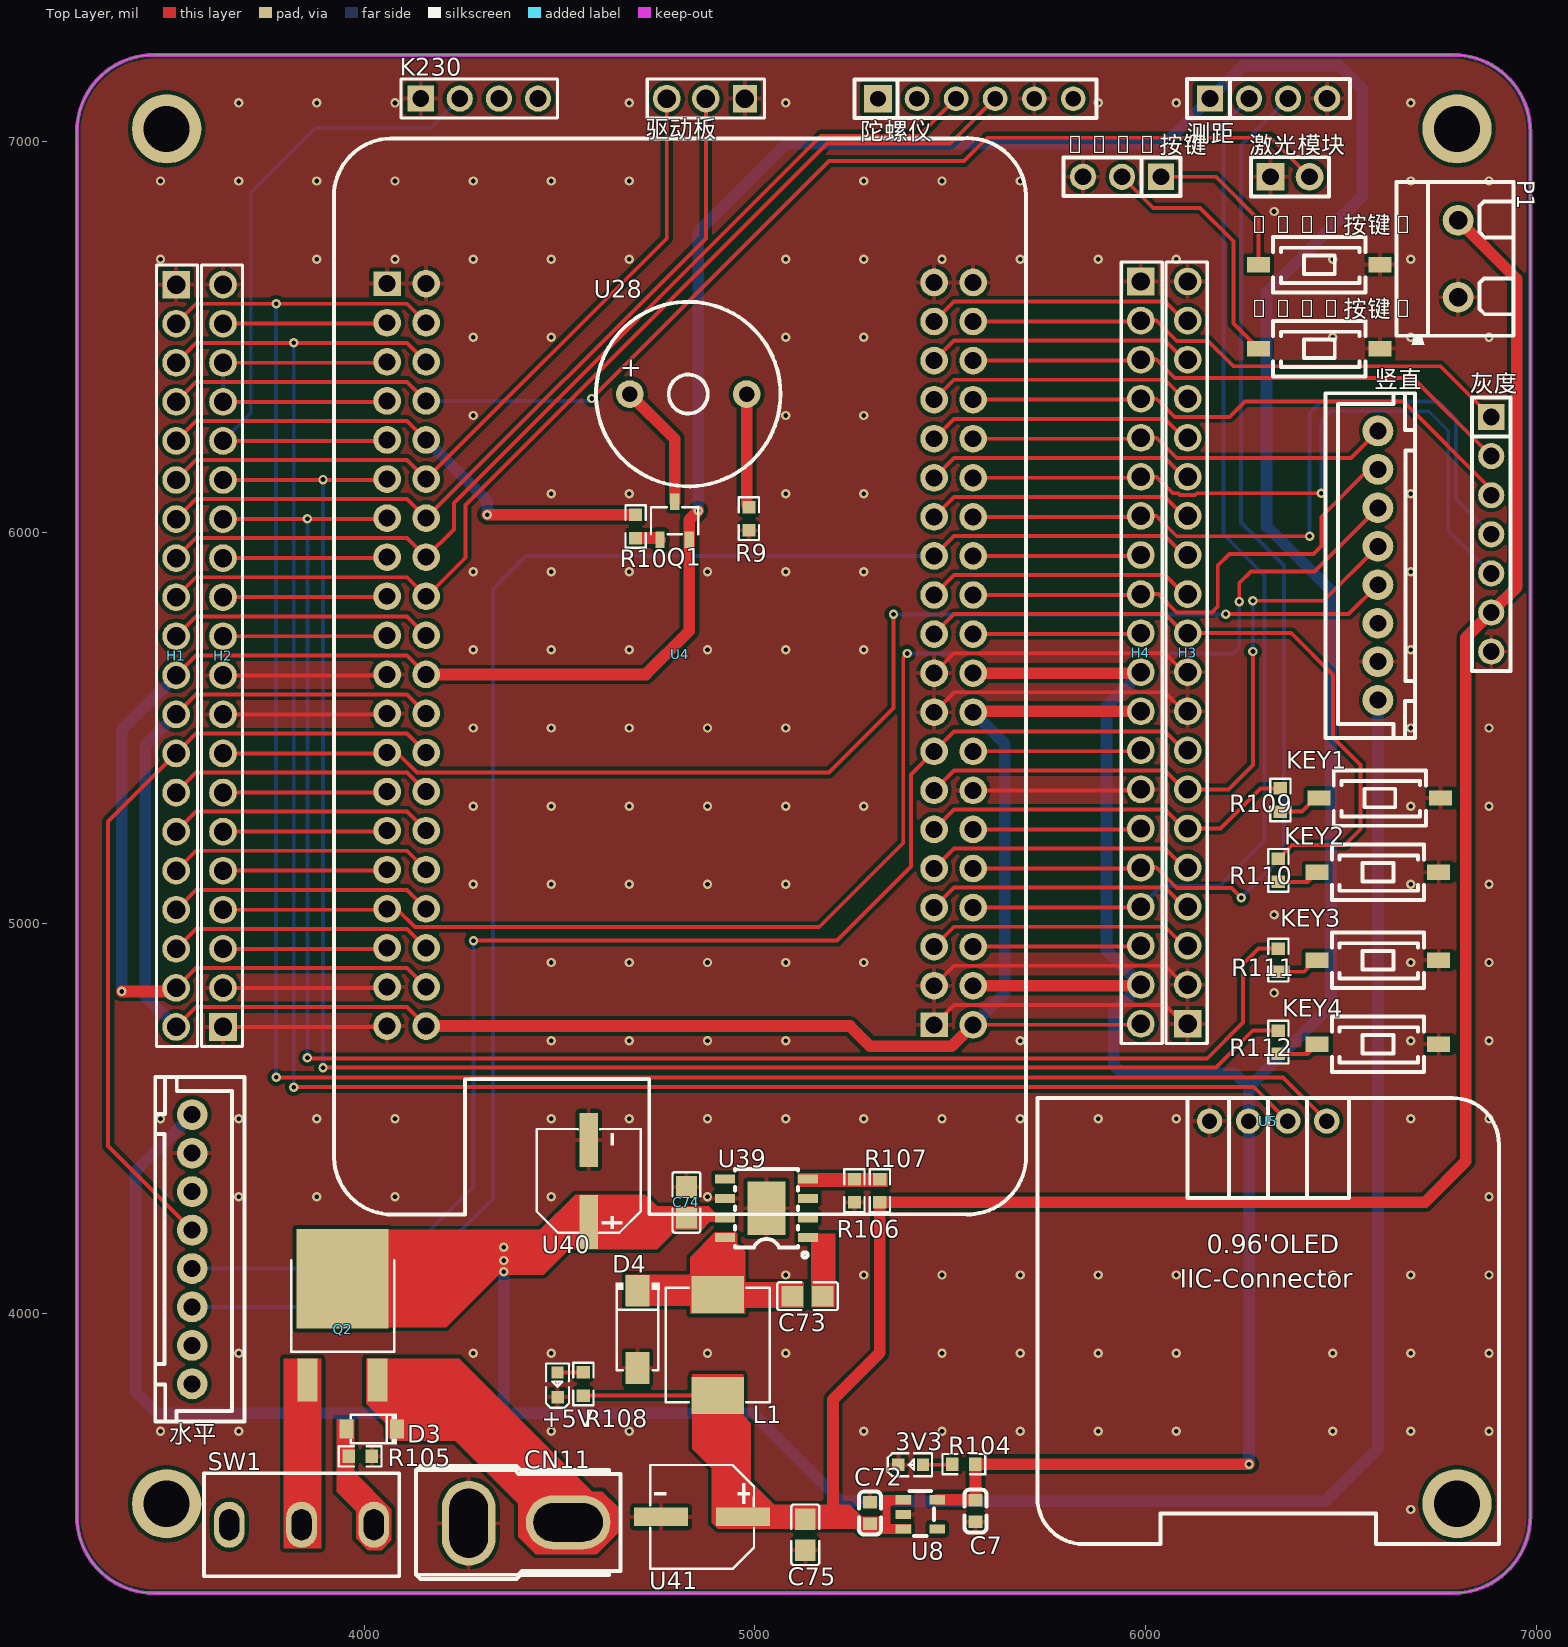
[diagram p0: Top Layer view]
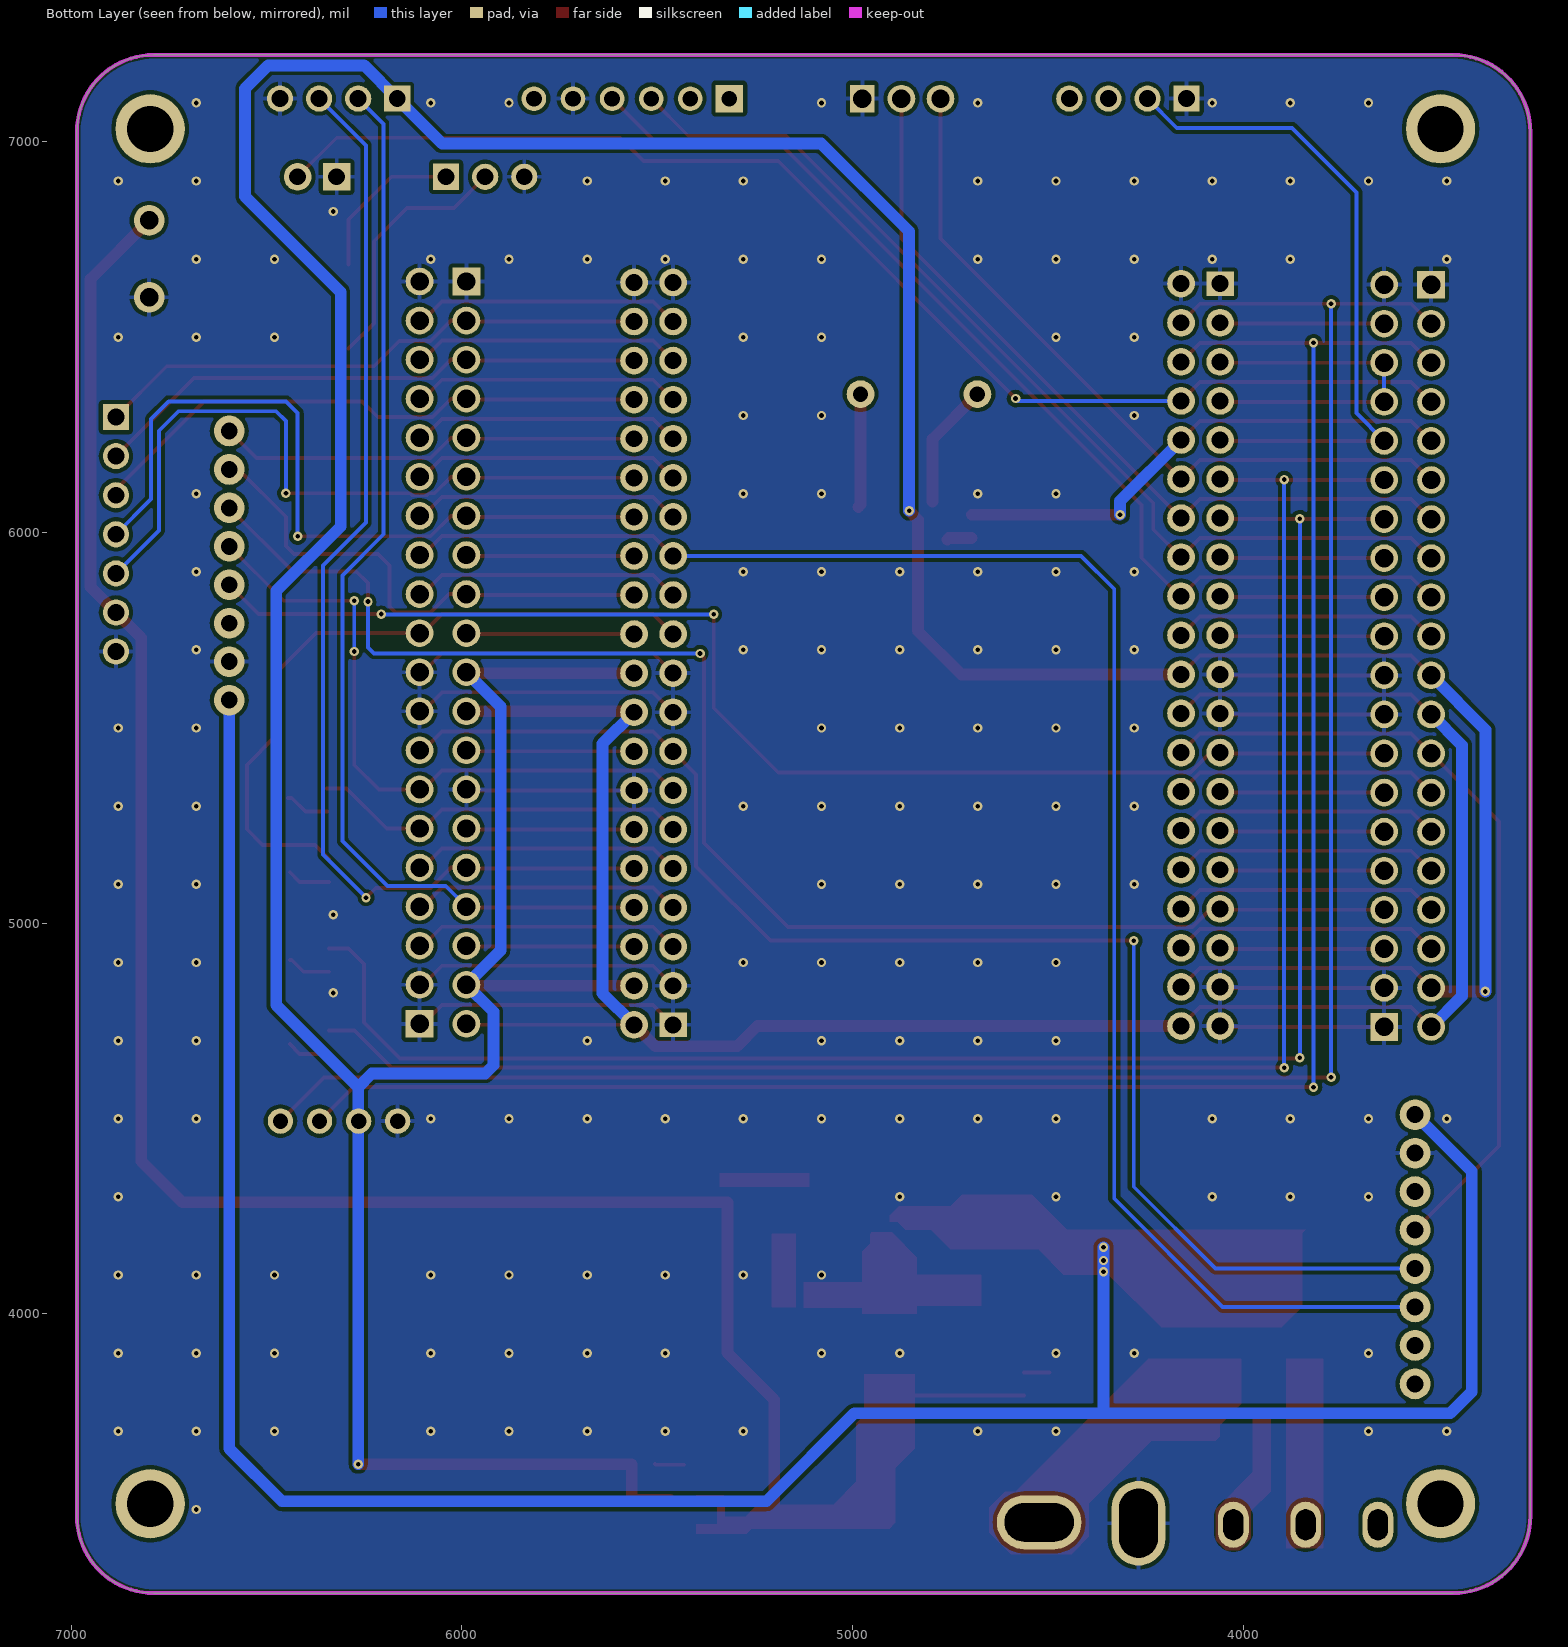
[diagram p1: Bottom Layer view, seen from below]
# Altium PCB MISC49883.pcbdoc
Units mil, origin at the board's own origin, x right, y up, seen from the top; angles counter-clockwise.
Board outline 3720 x 3937 mil, 2 copper layers (Top Layer, Bottom Layer), stack 62.206 mil thick; 52 components, 82 nets, 300 pads, 183 vias.

## Layer stack, top to bottom
Top Solder Mask Layer: solder mask 0.394, Dk 3.3
Top Layer: signal copper 1.379
Dielectric1: surface 59.449, FR4, Dk 4.5
Bottom Layer: signal copper 1.378
Bottom Solder Mask Layer: solder mask 0.394, Dk 3.3

## Board outline
3461.9,7222 ccw(c3461.9,7025.1) 3265,7025.1 3265,3481.9 ccw(c3461.9,3481.9) 3461.9,3285 6788.1,3285 ccw(c6788.1,3481.9) 6985,3481.9 6985,7025.1 ccw(c6788.1,7025.1) 6788.1,7222 3461.9,7222

## Design rules (kind name [scope] priority, off if disabled: settings)
BoardOutlineClearance copperThickness2oz_1 [All] p2 off: genericclearance=7.99 ignorepadtopadclearanceinfootprint=FALSE except(0: Arc-SplitContinuation Track-SplitContinuation SMDPad-SplitContinuation THPad-SplitContinuation Via-SplitContinuation Fill-SplitContinuation Region-SplitContinuation Poly-SplitContinuation Text-SplitContinuation Hole-SplitContinuation; 5.98: Arc-CutoutEdge Track-CutoutEdge SMDPad-CutoutEdge THPad-CutoutEdge Via-CutoutEdge Text-CutoutEdge; 6.9: Hole-OutlineEdge Hole-CutoutEdge; 10: Poly-OutlineEdge Poly-CutoutEdge; 11.81: Arc-OutlineEdge Track-OutlineEdge SMDPad-OutlineEdge THPad-OutlineEdge Via-OutlineEdge Fill-OutlineEdge Region-OutlineEdge Text-OutlineEdge Fill-CutoutEdge Region-CutoutEdge)
BoardOutlineClearance Plane_innerPlane_1 [All] p4 off: genericclearance=4.02 ignorepadtopadclearanceinfootprint=FALSE except(0: Arc-SplitContinuation Track-SplitContinuation SMDPad-SplitContinuation THPad-SplitContinuation Via-SplitContinuation Fill-SplitContinuation Region-SplitContinuation Poly-SplitContinuation Text-SplitContinuation Hole-SplitContinuation; 5.98: Arc-CutoutEdge Track-CutoutEdge SMDPad-CutoutEdge THPad-CutoutEdge Via-CutoutEdge Text-CutoutEdge; 6.9: Hole-OutlineEdge Hole-CutoutEdge; 10: Poly-OutlineEdge Poly-CutoutEdge; 11.81: Arc-OutlineEdge Track-OutlineEdge SMDPad-OutlineEdge THPad-OutlineEdge Via-OutlineEdge Fill-OutlineEdge Region-OutlineEdge Text-OutlineEdge Fill-CutoutEdge Region-CutoutEdge)
BoardOutlineClearance Copper_copperRegion_1 [All] p6 off: genericclearance=4.02 ignorepadtopadclearanceinfootprint=FALSE except(0: Arc-SplitContinuation Track-SplitContinuation SMDPad-SplitContinuation THPad-SplitContinuation Via-SplitContinuation Fill-SplitContinuation Region-SplitContinuation Poly-SplitContinuation Text-SplitContinuation Hole-SplitContinuation; 5.98: Arc-CutoutEdge Track-CutoutEdge SMDPad-CutoutEdge THPad-CutoutEdge Via-CutoutEdge Text-CutoutEdge; 6.9: Hole-OutlineEdge Hole-CutoutEdge; 10: Poly-OutlineEdge Poly-CutoutEdge; 11.81: Arc-OutlineEdge Track-OutlineEdge SMDPad-OutlineEdge THPad-OutlineEdge Via-OutlineEdge Fill-OutlineEdge Region-OutlineEdge Text-OutlineEdge Fill-CutoutEdge Region-CutoutEdge)
BoardOutlineClearance Copper_copperRegion_copperThickness1oz_1 [All] p8 off: genericclearance=4.02 ignorepadtopadclearanceinfootprint=FALSE except(0: Arc-SplitContinuation Track-SplitContinuation SMDPad-SplitContinuation THPad-SplitContinuation Via-SplitContinuation Fill-SplitContinuation Region-SplitContinuation Poly-SplitContinuation Text-SplitContinuation Hole-SplitContinuation; 5.98: Arc-CutoutEdge Track-CutoutEdge SMDPad-CutoutEdge THPad-CutoutEdge Via-CutoutEdge Text-CutoutEdge; 6.9: Hole-OutlineEdge Hole-CutoutEdge; 10: Poly-OutlineEdge Poly-CutoutEdge; 11.81: Arc-OutlineEdge Track-OutlineEdge SMDPad-OutlineEdge THPad-OutlineEdge Via-OutlineEdge Fill-OutlineEdge Region-OutlineEdge Text-OutlineEdge Fill-CutoutEdge Region-CutoutEdge)
BoardOutlineClearance Copper_copperRegion_Copper_copperRegion_1 [All] p10 off: genericclearance=4.02 ignorepadtopadclearanceinfootprint=FALSE except(0: Arc-SplitContinuation Track-SplitContinuation SMDPad-SplitContinuation THPad-SplitContinuation Via-SplitContinuation Fill-SplitContinuation Region-SplitContinuation Poly-SplitContinuation Text-SplitContinuation Hole-SplitContinuation; 5.98: Arc-CutoutEdge Track-CutoutEdge SMDPad-CutoutEdge THPad-CutoutEdge Via-CutoutEdge Text-CutoutEdge; 6.9: Hole-OutlineEdge Hole-CutoutEdge; 10: Poly-OutlineEdge Poly-CutoutEdge; 11.81: Arc-OutlineEdge Track-OutlineEdge SMDPad-OutlineEdge THPad-OutlineEdge Via-OutlineEdge Fill-OutlineEdge Region-OutlineEdge Text-OutlineEdge Fill-CutoutEdge Region-CutoutEdge)
BoardOutlineClearance copperThickness1oz_1 [All] p12: genericclearance=4.02 ignorepadtopadclearanceinfootprint=FALSE except(0: Arc-SplitContinuation Track-SplitContinuation SMDPad-SplitContinuation THPad-SplitContinuation Via-SplitContinuation Fill-SplitContinuation Region-SplitContinuation Poly-SplitContinuation Text-SplitContinuation Hole-SplitContinuation; 5.98: Arc-CutoutEdge Track-CutoutEdge SMDPad-CutoutEdge THPad-CutoutEdge Via-CutoutEdge Text-CutoutEdge; 6.9: Hole-OutlineEdge Hole-CutoutEdge; 10: Poly-OutlineEdge Poly-CutoutEdge; 11.81: Arc-OutlineEdge Track-OutlineEdge SMDPad-OutlineEdge THPad-OutlineEdge Via-OutlineEdge Fill-OutlineEdge Region-OutlineEdge Text-OutlineEdge Fill-CutoutEdge Region-CutoutEdge)
Clearance copperThickness2oz [All] p1 off: gap=7.99 ignorepadtopadclearanceinfootprint=FALSE except(5.98: SMDPad-Track SMDPad-SMDPad THPad-Track SMDPad-THPad THPad-THPad Track-Via SMDPad-Via THPad-Via Via-Via Fill-SMDPad Region-SMDPad Fill-THPad Region-THPad Fill-Via Region-Via Fill-Fill Fill-Region Region-Region Arc-Track Arc-SMDPad Arc-THPad Arc-Via Fill-Arc Region-Arc Arc-Arc Text-Track SMDPad-Text Text-THPad Text-Via Fill-Text Region-Text Arc-Text Text-Text; 6.9: Hole-Track Hole-SMDPad Hole-THPad Hole-Via Fill-Hole Region-Hole Hole-Arc Hole-Text; 10: Poly-Track Poly-SMDPad Poly-THPad Poly-Via Poly-Fill Poly-Region Poly-Poly Poly-Arc Poly-Text Poly-Hole; 11.81: Fill-Track Region-Track)
Clearance Plane_innerPlane [All] p3 off: gap=4.02 ignorepadtopadclearanceinfootprint=FALSE except(5.98: SMDPad-Track SMDPad-SMDPad THPad-Track SMDPad-THPad THPad-THPad Track-Via SMDPad-Via THPad-Via Via-Via Fill-SMDPad Region-SMDPad Fill-THPad Region-THPad Fill-Via Region-Via Fill-Fill Fill-Region Region-Region Arc-Track Arc-SMDPad Arc-THPad Arc-Via Fill-Arc Region-Arc Arc-Arc Text-Track SMDPad-Text Text-THPad Text-Via Fill-Text Region-Text Arc-Text Text-Text; 6.9: Hole-Track Hole-SMDPad Hole-THPad Hole-Via Fill-Hole Region-Hole Hole-Arc Hole-Text; 10: Poly-Track Poly-SMDPad Poly-THPad Poly-Via Poly-Fill Poly-Region Poly-Poly Poly-Arc Poly-Text Poly-Hole; 11.81: Fill-Track Region-Track)
Clearance Copper_copperRegion [All] p5 off: gap=4.02 ignorepadtopadclearanceinfootprint=FALSE except(5.98: SMDPad-Track SMDPad-SMDPad THPad-Track SMDPad-THPad THPad-THPad Track-Via SMDPad-Via THPad-Via Via-Via Fill-SMDPad Region-SMDPad Fill-THPad Region-THPad Fill-Via Region-Via Fill-Fill Fill-Region Region-Region Arc-Track Arc-SMDPad Arc-THPad Arc-Via Fill-Arc Region-Arc Arc-Arc Text-Track SMDPad-Text Text-THPad Text-Via Fill-Text Region-Text Arc-Text Text-Text; 6.9: Hole-Track Hole-SMDPad Hole-THPad Hole-Via Fill-Hole Region-Hole Hole-Arc Hole-Text; 10: Poly-Track Poly-SMDPad Poly-THPad Poly-Via Poly-Fill Poly-Region Poly-Poly Poly-Arc Poly-Text Poly-Hole; 11.81: Fill-Track Region-Track)
Clearance Copper_copperRegion_copperThickness1oz [All] p7 off: gap=4.02 ignorepadtopadclearanceinfootprint=FALSE except(5.98: SMDPad-Track SMDPad-SMDPad THPad-Track SMDPad-THPad THPad-THPad Track-Via SMDPad-Via THPad-Via Via-Via Fill-SMDPad Region-SMDPad Fill-THPad Region-THPad Fill-Via Region-Via Fill-Fill Fill-Region Region-Region Arc-Track Arc-SMDPad Arc-THPad Arc-Via Fill-Arc Region-Arc Arc-Arc Text-Track SMDPad-Text Text-THPad Text-Via Fill-Text Region-Text Arc-Text Text-Text; 6.9: Hole-Track Hole-SMDPad Hole-THPad Hole-Via Fill-Hole Region-Hole Hole-Arc Hole-Text; 10: Poly-Track Poly-SMDPad Poly-THPad Poly-Via Poly-Fill Poly-Region Poly-Poly Poly-Arc Poly-Text Poly-Hole; 11.81: Fill-Track Region-Track)
Clearance Copper_copperRegion_Copper_copperRegion [All] p9 off: gap=4.02 ignorepadtopadclearanceinfootprint=FALSE except(5.98: SMDPad-Track SMDPad-SMDPad THPad-Track SMDPad-THPad THPad-THPad Track-Via SMDPad-Via THPad-Via Via-Via Fill-SMDPad Region-SMDPad Fill-THPad Region-THPad Fill-Via Region-Via Fill-Fill Fill-Region Region-Region Arc-Track Arc-SMDPad Arc-THPad Arc-Via Fill-Arc Region-Arc Arc-Arc Text-Track SMDPad-Text Text-THPad Text-Via Fill-Text Region-Text Arc-Text Text-Text; 6.9: Hole-Track Hole-SMDPad Hole-THPad Hole-Via Fill-Hole Region-Hole Hole-Arc Hole-Text; 10: Poly-Track Poly-SMDPad Poly-THPad Poly-Via Poly-Fill Poly-Region Poly-Poly Poly-Arc Poly-Text Poly-Hole; 11.81: Fill-Track Region-Track)
Clearance copperThickness1oz [All] p11: gap=4.02 ignorepadtopadclearanceinfootprint=FALSE except(5.98: SMDPad-Track SMDPad-SMDPad THPad-Track SMDPad-THPad THPad-THPad Track-Via SMDPad-Via THPad-Via Via-Via Fill-SMDPad Region-SMDPad Fill-THPad Region-THPad Fill-Via Region-Via Fill-Fill Fill-Region Region-Region Arc-Track Arc-SMDPad Arc-THPad Arc-Via Fill-Arc Region-Arc Arc-Arc Text-Track SMDPad-Text Text-THPad Text-Via Fill-Text Region-Text Arc-Text Text-Text; 6.9: Hole-Track Hole-SMDPad Hole-THPad Hole-Via Fill-Hole Region-Hole Hole-Arc Hole-Text; 10: Poly-Track Poly-SMDPad Poly-THPad Poly-Via Poly-Fill Poly-Region Poly-Poly Poly-Arc Poly-Text Poly-Hole; 11.81: Fill-Track Region-Track)
DiffPairsRouting differentialPair [All] p1: maxlimit=6 minlimit=6 mostfreqgap=6 toplayer_minwidth=5 toplayer_prefwidth=10 toplayer_maxwidth=100 toplayer_mingap=6 toplayer_prefgap=6 toplayer_maxgap=6 bottomlayer_minwidth=5 bottomlayer_prefwidth=10 bottomlayer_maxwidth=100 bottomlayer_mingap=6 bottomlayer_prefgap=6 bottomlayer_maxgap=6 maxuncoupledlength=10
HoleToHoleClearance otherClearance [All] p1: gap=11.81 allowstackedmicrovias=TRUE
Length netLength [All] p1: minlimit=0 maxlimit=0
PasteMaskExpansion pasteMaskExpansion [All] p1: expansion=0
PlaneConnect innerPlane [All] p1: planeconnectstyle=Relief reliefexpansion=20 reliefentries=4 reliefconductorwidth=10 reliefairgap=10
PolygonConnect copperRegion_copperThickness1oz [All] p1 off: connectstyle=Relief reliefconductorwidth=10 reliefentries=4 polygonreliefangle="90 Angle" airgapwidth=10 via.connectstyle=Relief via.reliefconductorwidth=10 via.reliefentries=4 via.polygonreliefangle="90 Angle" via.airgapwidth=10
PolygonConnect copperRegion_Copper_copperRegion [All] p2 off: connectstyle=Relief reliefconductorwidth=10 reliefentries=4 polygonreliefangle="90 Angle" airgapwidth=10 via.connectstyle=Relief via.reliefconductorwidth=10 via.reliefentries=4 via.polygonreliefangle="90 Angle" via.airgapwidth=10
PolygonConnect copperRegion [All] p3: connectstyle=Relief reliefconductorwidth=10 reliefentries=4 polygonreliefangle="90 Angle" airgapwidth=10 via.connectstyle=Relief via.reliefconductorwidth=10 via.reliefentries=4 via.polygonreliefangle="90 Angle" via.airgapwidth=10
RoutingVias viaSize [All] p1: holewidth=12.01 width=24.02 viastyle="Through Hole" minholewidth=11.81 minwidth=19.68 maxholewidth=248.03 maxwidth=393.7
SolderMaskExpansion solderMaskExpansion [IsVia] p1: expansion=-1000 istentingtop=TRUE
SolderMaskExpansion solderMaskExpansion [All] p2: expansion=2 istentingtop=FALSE
Width copperThickness2oz_2 [All] p1 off: maxlimit=100 minlimit=8 preferedwidth=10
Width copperThickness1oz_2 [All] p2: maxlimit=100 minlimit=5 preferedwidth=10

## Components (designator, comment, footprint, x,y, rotation, side; value= is the part's Value field where it differs from the comment)
3V3 "" LED_0603 5401.02,3613.64 r0 top
+5V "" LED_0603 4495,3820 r90 top
C7 "1uF" C0603 5565,3495 r90 top
C72 "1uF" C0603 5295,3490 r270 top
C73 "100nF" C0805 5135,4045 r180 top
C74 "100nF" C0805 4825,4285 r270 top
C75 "100nF" C0805 5129.37,3434.37 r90 top
CN11 "AM-1015B-M" CONN-TH_AM-1015B-M 4395,3465 r0 top
D3 "BZT52C16" SOD-123_L2.7-W1.6-LS3.7-RD 4020,3705 r180 top
D4 "SS54" SMA_L4.4-W2.8-LS5.4-R-RD 4700,3960 r270 top
H1 "" HDR-TH_20P-P2.54-V-M-1 3519,5684 r270 top
H2 "" HDR-TH_20P-P2.54-V-M-1 3639,5684 r90 top
H3 "" HDR-TH_20P-P2.54-V-M-1 6108,5692 r90 top
H4 "" HDR-TH_20P-P2.54-V-M-1 5988,5692 r270 top
K230 "2.54*4 single row" HDR-TH_4P-P2.54-V-M-1 4295,7110 r0 top
K230按键 "K230 button" HDR-TH_3P-P2.54-V-M 5940,6910 r180 top
K230按键1 "Tact switch 3*6*2.5" SW-SMD_L6.0-W3.6-LS8.0 6445,6685 r0 top
K230按键2 "Tact switch 3*6*2.5" SW-SMD_L6.0-W3.6-LS8.0 6445,6470 r0 top
KEY1 "Tact switch 3*6*2.5" SW-SMD_L6.0-W3.6-LS8.0 6600,5320 r0 top
KEY2 "Tact switch 3*6*2.5" SW-SMD_L6.0-W3.6-LS8.0 6595,5130 r0 top
KEY3 "Tact switch 3*6*2.5" SW-SMD_L6.0-W3.6-LS8.0 6595,4905 r0 top
KEY4 "Tact switch 3*6*2.5" SW-SMD_L6.0-W3.6-LS8.0 6595,4690 r0 top
L1 "4.7uH" IND-SMD_L7.3-W6.6 4905,3920 r90 top
P1 "KF301-2P terminal block" CONN-TH_XY301V-A-5.0-2P 6800,6700 r270 top
Q1 "S8550" SOT-23-3_L2.9-W1.6-P1.90-LS2.8-BR 4795,6030 r270 top
Q2 "HY19P03D" TO-252-2_L6.6-W6.1-P4.57-LS9.9-TL-CW 3945,3960 r90 top
R9 "100Ω" R0603 4985,6035 r90 top
R10 "100Ω" R0603 4695,6015 r90 top
R104 "10K" R0603 5535,3615 r180 top
R105 "10kΩ" R0603 3990,3635 r180 top
R106 "3.24K" R0603 5255,4315 r90 top
R107 "10K" R0603 5320,4315 r270 top
R108 "4.7K" R0603 4561.29,3820.26 r270 top
R109 "100Ω" R0603 6345,5315 r90 top
R110 "100Ω" R0603 6340,5135 r90 top
R111 "100Ω" R0603 6340,4905 r90 top
R112 "100Ω" R0603 6340,4695 r90 top
SW1 "SS-12D10L5" SW-TH_SS-12D10L5 3840,3460 r180 top
U4 "" COMM-TH_LCKFB-TMX-MSPM0G3507 4809,5688 r0 top
U5 "" 0.96OLED_4P 6314,4493 r0 top
U8 "TLV75733PDBVR" SOT-23-5_L2.9-W1.6-P0.95-LS2.8-BL 5423.52,3486.48 r270 top
U28 "2.6kHz" BUZ-TH_BD12.0-P7.60-D0.6-FD 4829.7,6353.8 r0 top
U39 "TPS5430DDAR" ESOP-8_L4.9-W3.9-P1.27-LS6.0-TL-EP 5030,4270 r180 top
U40 "220uF" CAP-SMD_BD6.3-L6.6-W6.6-LS7.2-FD 4575,4340 r90 top
U41 "220uF" CAP-SMD_BD6.3-L6.6-W6.6-LS7.2-FD 4865,3480 r180 top
水平 "Horizontal" CONN-TH_8P-P2.50-XH2.54-8P 3560,4165 r90 top (schematic designator ˮƽ)
测距 "PM2.54-1*4" HDR-TH_4P-P2.54-V-F 6315,7110 r0 top
激光模块 "" HDR-TH_2P-P2.54-V-M-1 6370,6910 r0 top
灰度 "PZ2.54-1*7" HDR-TH_7P-P2.54-V-M 6885,5995 r270 top
竖直 "Vertical" CONN-TH_8P-P2.50-XH2.54-8P 6595,5915 r270 top
陀螺仪 "2.54-1*6P female" HDR-TH_6P-P2.54-V-F 5565.21,7110 r0 top
驱动板 "2.54mm-1*3P straight pin" HDR-TH_3P-P2.54-V-M-1 4874.68,7110 r180 top

## Footprints (in the part's own frame and the unit in brackets; to place one, negate y for a bottom-side part, rotate by r counter-clockwise, add the part's x,y. Pads: shape width x height; smd on the part's side, far side on the other; paste and mask are expansions set on the pad)
0.96OLED_4P [mm]
  round 1.65 hole 1 copper offset 0,0: 1(-3.81,-0.001) 2(-1.27,0.002) 3(1.27,0.002) 4(3.81,0.002)
  silkscreen extent -15,-27.5 15,1.5
BUZ-TH_BD12.0-P7.60-D0.6-FD [mm]
  round 1.8 hole 1: 1(-3.8,0) 2(3.8,0)
  silkscreen extent -6,-6 6,6
C0603 [mm]
  rect 0.8x0.9 smd: 1(-0.7,0) 2(0.7,0)
  silkscreen extent -1.39,-0.71 1.39,0.71
C0805 [mm]
  rect 1.41x1.35 smd paste-100 mask+0.051: 1(-1,0) 2(1,0)
  silkscreen extent -1.96,-0.9 1.96,0.9
CAP-SMD_BD6.3-L6.6-W6.6-LS7.2-FD [mm]
  rect 3.5x1.2 smd: 1(-2.67,0) 2(2.67,0)
  silkscreen extent -3.38,-3.38 3.38,3.38
COMM-TH_LCKFB-TMX-MSPM0G3507 [mm]
  rect 1.8x1.575 hole 1.1: 1(-19.05,24.09) 41(16.51,-24.09)
  round 1.8 hole 1.1: 2(-16.51,24.09) 3(-19.05,21.55) 4(-16.51,21.55) 5(-19.05,19.01) 6(-16.51,19.01) 7(-19.05,16.47) 8(-16.51,16.47) 9(-19.05,13.93) 10(-16.51,13.93) 11(-19.05,11.39) 12(-16.51,11.39) 13(-19.05,8.85) 14(-16.51,8.85) 15(-19.05,6.31) 16(-16.51,6.31) 17(-19.05,3.77) 18(-16.51,3.77) 19(-19.05,1.23) 20(-16.51,1.23) 21(-19.05,-1.31) 22(-16.51,-1.31) 23(-19.05,-3.85) 24(-16.51,-3.85) 25(-19.05,-6.39) 26(-16.51,-6.39) 27(-19.05,-8.93) 28(-16.51,-8.93) 29(-19.05,-11.47) 30(-16.51,-11.47) 31(-19.05,-14.01) 32(-16.51,-14.01) 33(-19.05,-16.55) 34(-16.51,-16.55) 35(-19.05,-19.09) 36(-16.51,-19.09) 37(-19.05,-21.63) 38(-16.51,-21.63) 39(-19.05,-24.17) 40(-16.51,-24.17) 42(19.05,-24.09) 43(16.51,-21.55) 44(19.05,-21.55) 45(16.51,-19.01) 46(19.05,-19.01) 47(16.51,-16.47) 48(19.05,-16.47) 49(16.51,-13.93) 50(19.05,-13.93) 51(16.51,-11.39) 52(19.05,-11.39) 53(16.51,-8.85) 54(19.05,-8.85) 55(16.51,-6.31) 56(19.05,-6.31) 57(16.51,-3.77) 58(19.05,-3.77) 59(16.51,-1.23) 60(19.05,-1.23) 61(16.51,1.31) 62(19.05,1.31) 63(16.51,3.85) 64(19.05,3.85) 65(16.51,6.39) 66(19.05,6.39) 67(16.51,8.93) 68(19.05,8.93) 69(16.51,11.47) 70(19.05,11.47) 71(16.51,14.01) 72(19.05,14.01) 73(16.51,16.55) 74(19.05,16.55) 75(16.51,19.09) 76(19.05,19.09) 77(16.51,21.63) 78(19.05,21.63) 79(16.51,24.17) 80(19.05,24.17)
  silkscreen extent -22.52,-36.43 22.49,33.55
CONN-TH_8P-P2.50-XH2.54-8P [mm]
  round 2 hole 1.1: 1(8.75,0) 2(6.25,0) 3(3.75,0) 4(1.25,0) 5(-1.25,0) 6(-3.75,0) 7(-6.25,0) 8(-8.75,0)
  silkscreen extent -11.2,-3.4 11.2,2.4
CONN-TH_AM-1015B-M [mm]
  oval 3.5x5.5 hole 2.5 slot 4.5 at 90 deg: 1(-3.231,-0.029)
  oval 5.5x3.5 hole 2.5 slot 4.5 at 0 deg: 2(3.231,0.029)
  silkscreen extent -6.65,-3.65 6.65,3.68
CONN-TH_XY301V-A-5.0-2P [mm]
  round 2 hole 1.2: 1(-2.5,0) 2(2.5,0)
  silkscreen extent -5,-4 5.6,3.6
ESOP-8_L4.9-W3.9-P1.27-LS6.0-TL-EP [mm]
  rect 1.3x0.6 smd: 1(-2.7,1.905) 2(-2.7,0.635) 3(-2.7,-0.635) 4(-2.7,-1.905) 5(2.7,-1.905) 6(2.7,-0.635) 7(2.7,0.635) 8(2.7,1.905)
  rect 2.5x3.5 smd: 9(0,0)
  silkscreen extent -2.67,-2.55 2.05,3.2
HDR-TH_2P-P2.54-V-M-1 [mm]
  rect 1.8x1.8 hole 1.1: 1(-1.27,0)
  round 1.8 hole 1.1: 2(1.27,0)
  silkscreen extent -2.54,-1.27 2.54,1.27
HDR-TH_3P-P2.54-V-M [mm]
  rect 1.7x1.7 hole 1.1: 1(-2.54,0)
  round 1.7 hole 1.1: 2(0,0) 3(2.54,0)
  silkscreen extent -3.81,-1.25 3.81,1.25
HDR-TH_3P-P2.54-V-M-1 [mm]
  rect 1.575x1.8 hole 1.2: 1(-2.54,0)
  round 1.8 hole 1.2: 2(0,0) 3(2.54,0)
  silkscreen extent -3.81,-1.27 3.81,1.27
HDR-TH_4P-P2.54-V-F [mm]
  rect 1.7x1.7 hole 1.1: 1(-3.81,0)
  round 1.7 hole 1.1: 2(-1.27,0) 3(1.27,0) 4(3.81,0)
  silkscreen extent -5.29,-1.27 5.29,1.27
HDR-TH_4P-P2.54-V-M-1 [mm]
  rect 1.7x1.7 hole 1.1: 1(-3.81,0)
  round 1.7 hole 1.1: 2(-1.27,0) 3(1.27,0) 4(3.81,0)
  silkscreen extent -5.08,-1.27 5.08,1.27
HDR-TH_6P-P2.54-V-F [mm]
  rect 1.8x1.8 hole 1.02: 1(-6.35,0)
  round 1.6 hole 1.02: 2(-3.81,0) 3(-1.27,0) 4(1.27,0) 5(3.81,0) 6(6.35,0)
  silkscreen extent -7.87,-1.25 7.87,1.25
HDR-TH_7P-P2.54-V-M [mm]
  rect 1.7x1.7 hole 1.1: 1(-7.62,0)
  round 1.7 hole 1.1: 2(-5.08,0) 3(-2.54,0) 4(0,0) 5(2.54,0) 6(5.08,0) 7(7.62,0)
  silkscreen extent -8.89,-1.25 8.89,1.25
HDR-TH_20P-P2.54-V-M-1 [mm]
  rect 1.8x1.8 hole 1.2: 1(-24.13,0)
  round 1.8 hole 1.2: 2(-21.59,0) 3(-19.05,0) 4(-16.51,0) 5(-13.97,0) 6(-11.43,0) 7(-8.89,0) 8(-6.35,0) 9(-3.81,0) 10(-1.27,0) 11(1.27,0) 12(3.81,0) 13(6.35,0) 14(8.89,0) 15(11.43,0) 16(13.97,0) 17(16.51,0) 18(19.05,0) 19(21.59,0) 20(24.13,0)
  silkscreen extent -25.4,-1.27 25.4,1.4
IND-SMD_L7.3-W6.6 [mm]
  rect 2.424x3.42 smd: 1(3.278,0) 2(-3.278,0)
  silkscreen extent -3.73,-3.38 3.73,3.38
LED_0603 [mil]
  rect 31.5x31.5 smd paste+0 mask+2: 1(-33.5,-0.4) 2(29.5,-0.2)
  silkscreen extent -61,-30 53,30
R0603 [mil]
  rect 31.75x34.02 smd paste-3937.01 mask+2: 1(-29.66,0) 2(29.66,0)
  silkscreen extent -55,-26 55,26
SMA_L4.4-W2.8-LS5.4-R-RD [mil]
  rect 81.2x60.59 smd: 1(98.57,0) 2(-98.57,0)
  silkscreen extent -119,-56 104,56
SOD-123_L2.7-W1.6-LS3.7-RD [mm]
  rect 0.91x1.22 smd: 1(-1.635,0) 2(1.635,0)
  silkscreen extent -1.6,-1 1.38,1
SOT-23-3_L2.9-W1.6-P1.90-LS2.8-BR [mm]
  rect 1.07x0.6 smd: 1(1.235,-0.95) 2(1.235,0.95) 3(-1.235,0)
  silkscreen extent -0.88,-1.54 0.88,1.54
SOT-23-5_L2.9-W1.6-P0.95-LS2.8-BL [mm]
  rect 0.6x1 smd paste+0 mask+0.05: 1(-0.95,-1.1) 2(0,-1.1) 3(0.95,-1.1) 4(0.95,1.1) 5(-0.95,1.1)
  silkscreen extent -1.52,-0.7 1.4,0.89
SW-SMD_L6.0-W3.6-LS8.0 [mm]
  rect 1.5x1 smd: 1(-3.95,0) 2(3.95,0)
  silkscreen extent -3,-1.8 3,1.8
SW-TH_SS-12D10L5 [mm]
  oval 2x3 hole 1.3 slot 2 at 90 deg: 1(-4.7,0) 2(0,0) 3(4.7,0)
  silkscreen extent -6.35,-3.35 6.35,3.35
TO-252-2_L6.6-W6.1-P4.57-LS9.9-TL-CW [mm]
  rect 2.8x1.3 smd: 1(-3.292,2.273) 3(-3.292,-2.273)
  rect 6.5x6 smd: 2(3.292,0)
  silkscreen extent -1.46,-3.35 4.51,3.34

## Free pads (board coordinates)
  round 177.2 hole 118.1: 1(3494.7,7032.7) 2(6797.4,7032.7) 3(3494.7,3513.7) 4(6797.4,3513.7)

## Via types
v1: diameter 24.02, hole 12, Top Layer to Bottom Layer, 183 vias

## Nets (pads, with @x,y where several pads share a name; then routed paths per layer and width w, separated by ;. In a path a pad name is that pad's centre, name@x,y a point inside that pad or via, vN(x,y) a via of type N, cw(c..) or ccw(c..) an arc to the next point about the centre after c; other vN are vias at no path point)
3.3V: 陀螺仪.2
3V3: C7.2 H1.11 H1.19 H4.11 H4.19 Q1.2 R104.1 U4.22 U4.38 U4.44 U4.60 U5.2 U8.5 测距.1 | length 13030.8
  Top Layer w10: H1.19 3570,4885 4110.41,4885 U4.38 ; H1.11 3570,5685 4110.41,5685 U4.22
  Top Layer w30: v1(3380,4825) 3510,4825 H1.19 ; U4.22 4721.41,5636.41 4832.4,5747.4 Q1.2 4832.4,6032.4 v1(4855,6055) ; U8.5 5563.68,3523.88 C7.2 5565,3614.66 R104.1 v1(6265,3615) ; U4.44 5985.59,4839.59 H4.19 ; U4.60 5985.59,5639.59 H4.11
  Bottom Layer w30: v1(3380,4825) 3380,5495 H1.11 ; v1(4855,6055) 4855,6770 5080,6995 6050,6995 测距.1 6250,7195 6495,7195 6555,7135 6555,6860 6310,6615 6310,6015 6475,5850 6475,4790 6265,4580 ; H4.11 5900,5554 5900,4930 H4.19 5918.79,4772.79 5918.79,4636.21 5940,4615 6230,4615 6265,4580 ; U5.2@6264,4493.05 U5.2@6265,4492.05 ; v1(6265,3615) U5.2@6265,4492.05 ; U5.2@6265,4492.05 6265,4580
5V: H1.12 H1.20 H4.12 H4.20 U4.24 U4.40 U4.42 U4.58 | length 5393.4
  Top Layer w10: H1.20 3570,4785 4110.41,4785 U4.40 ; H1.12 3570,5585 4110.41,5585 U4.24 ; U4.42@5579,4739.59 5996.59,4739.59 H4.20@5999,4742 ; H4.12@5996.59,5539.59 H4.12@5999,5542
  Top Layer w30: U4.40 5243.59,4736.41 5295,4685 5504.41,4685 U4.42 ; U4.58 5561.41,5542 H4.12
  Bottom Layer w30: H1.20 3440,4813 3440,5455 H1.12 ; U4.42 5640,4820.59 5640,5458.59 U4.58
12V: C74.2 Q2.2 U39.7 U40.1 水平.1 竖直.1 | length 6462
  Bottom Layer w30: 水平.1 3415,4364.49 3415,3800 3470,3745 4357.33,3745 ; v1(4357.33,4170) v1(4357.33,4136.19) v1(4357.33,4107.32) 4357.33,3745 ; 竖直.1 6595,3655 6460,3520 5220,3520 4995,3745 4357.33,3745
$1N1506: 3V3.2 R104.2 | length 75.5
  Top Layer w10: 3V3.2 5503.78,3613.44 R104.2
$1N2883: H2.11 U4.19 | length 421
  Top Layer w10: H2.11 4056.59,5734 U4.19
$1N2891: H2.3 U4.35 | length 421
  Top Layer w10: H2.3 4056.59,4934 U4.35
$1N2924: H1.18 U4.36 | length 681.3
  Top Layer w10: H1.18 3570,4985 4110.41,4985 U4.36
$1N2927: H1.10 U4.20 | length 681.3
  Top Layer w10: H1.10 3570,5785 4110.41,5785 U4.20
$1N3031: H3.3 U4.45 | length 681.3
  Top Layer w10: U4.45 5510,4990.59 6050.41,4990.59 H3.3@6099,4942
$1N6236: Q1.3 U28.1 | length 322.8
  Top Layer w30: U28.1 4795,6238.9 Q1.3
$1N6238: Q1.1 R10.1 | length 64.2
  Top Layer w30: R10.1 4753.64,5985.34 Q1.1
$1N6240: R9.2 U28.2 | length 291.5
  Top Layer w30: U28.2 4979.31,6070.35 R9.2
$1N19638: CN11.2 D3.1 Q2.3
$1N19825: D3.2 R105.2 SW1.1
$1N19859: Q2.1 SW1.2
$1N23197: C73.1 U39.1
$1N23203: C73.2 D4.2 L1.1 U39.8
$1N23919: +5V.2 R108.1 | length 66.3
  Top Layer w10: +5V.2 4560.86,3849.5 R108.1
$1N33683: KEY1.1 R109.1 | length 113.8
  Top Layer w10: R109.1 6400.34,5285.34 6435,5320 KEY1.1
$1N33684: KEY2.1 R110.1 | length 109.7
  Top Layer w10: R110.1 6414.83,5105.34 KEY2.1
$1N33685: KEY3.1 R111.1 | length 111.8
  Top Layer w10: R111.1 6405.34,4875.34 6435,4905 KEY3.1
$1N33686: KEY4.1 R112.1 | length 109.7
  Top Layer w10: R112.1 6414.83,4665.34 KEY4.1
$1N37357: R106.2 R107.1 U39.4
+5V: C72.2 C75.2 L1.2 P1.1 R107.2 R108.2 U8.1 U8.3 U41.1 灰度.6 | length 5271.6
  Top Layer w10: R108.2 4904.67,3790.61 L1.2
  Top Layer w30: 5200,3475 5200,3780 5320,3900 R107.2 6715.34,4285.34 6820,4390 6820,5730 灰度.6 6950,5860 6950,6648.43 P1.1
BUZZER: H1.5 R10.2 U4.10 | length 1317.4
  Top Layer w10: H1.5 3570,6285 4110.41,6285 U4.10
  Top Layer w30: v1(4315,6045) 4315.34,6044.66 R10.2
  Bottom Layer w30: U4.10 4315,6080.41 v1(4315,6045)
DIR1: H3.13 U4.65 水平.6 | length 4290.3
  Top Layer w10: U4.65 5510,5990.59 6050.41,5990.59 H3.13@6099,5942
  Bottom Layer w10: 水平.6 4052.36,4017.36 4330,4295 4330,5855 4414.59,5939.59 U4.65
DIR2: H2.4 U4.33 竖直.6 | length 3795.4
  Top Layer w10: H2.4 4056.59,5034 U4.33 4083.59,5036.41 4130,4990 5165,4990 5380,5205 5380,5680 v1(5390,5690) ; v1(6240,5822.8) 6240,5870 6270,5900 6432.36,5900 竖直.6
  Bottom Layer w10: v1(5390,5690) 6225,5690 6240,5705 v1(6240,5822.8)
ECHO: H4.16 U4.50 测距.3 | length 2895.7
  Top Layer w10: U4.50@5579,5139.59 5996.59,5139.59 H4.16@5999,5142 ; H4.16 H4.16@5999,5142 ; v1(6245,5065) 6220,5090 6080,5090 6028,5142 H4.16@5999,5142
  Bottom Layer w10: v1(6245,5065) 6355,5175 6355,5915 6245,6025 6245,6990 测距.3
EN1: H1.13 U4.26 水平.4 | length 2062.2
  Top Layer w10: 水平.4 3345,4429.21 3345,5260 H1.13 3570,5485 4110.41,5485 U4.26
EN2: H2.8 U4.25 竖直.4 | length 3318
  Top Layer w10: H2.8 4056.59,5434 U4.25 4083.59,5436.41 4135,5385 5190,5385 5355,5550 v1(5355,5790) ; v1(6205.79,5790.79) 6520,5790.79 竖直.4
  Bottom Layer w10: v1(5355,5790) 6205,5790 v1(6205.79,5790.79)
GND: 3V3.1 +5V.1 C7.1 C72.1 C74.1 C75.1 CN11.1 D4.1 H1.1 H2.1 H2.2 H2.9 H2.10 H2.20 H3.1 H3.2 H3.9 H3.10 H3.20 H4.1 H4.14 K230.1 K230按键1.2 K230按键2.2 K230按键.3 KEY1.2 KEY2.2 KEY3.2 KEY4.2 P1.2 R9.1 R105.1 R106.1 U4.1 U4.2 U4.21 U4.23 U4.37 U4.39 U4.41 U4.43 U4.54 U4.57 U4.59 U4.79 U4.80 U5.1 U8.2 U39.6 U39.9 U40.2 U41.2 水平.2 测距.4 激光模块.1 灰度.7 竖直.2 陀螺仪.5 驱动板.1 | length 4830
  Top Layer w10: H2.1 4056.59,4734 U4.39 ; H2.2 4056.59,4834 U4.37 ; H2.9 4056.59,5534 U4.23 ; H2.10 4056.59,5634 U4.21 ; U4.41 5510,4790.59 6050.41,4790.59 H3.1@6099,4742 ; U4.43 5510,4890.59 6050.41,4890.59 H3.2@6099,4842 ; U4.57 5510,5590.59 6050.41,5590.59 H3.9@6099,5542 ; U4.59 5510,5690.59 6050.41,5690.59 H3.10@6099,5642 ; U4.54@5579,5339.59 5996.59,5339.59 H4.14@5999,5342
  other v1: 6679.1,3499.1 3479.1,3699.1 3679.1,3699.1 4479.1,3699.1 4679.1,3699.1 5279.1,3699.1 5479.1,3699.1 5679.1,3699.1 5879.1,3699.1 6079.1,3699.1 6479.1,3699.1 6679.1,3699.1 6879.1,3699.1 3679.1,3899.1 4279.1,3899.1 4479.1,3899.1 4879.1,3899.1 5079.1,3899.1 5479.1,3899.1 5679.1,3899.1 5879.1,3899.1 6079.1,3899.1 6479.1,3899.1 6679.1,3899.1 6879.1,3899.1 5079.1,4099.1 5279.1,4099.1 5479.1,4099.1 5679.1,4099.1 5879.1,4099.1 6079.1,4099.1 6479.1,4099.1 6679.1,4099.1 6879.1,4099.1 3679.1,4299.1 3879.1,4299.1 4079.1,4299.1 4479.1,4299.1 4879.1,4299.1 6879.1,4299.1 3479.1,4499.1 3679.1,4499.1 3879.1,4499.1 4079.1,4499.1 4479.1,4499.1 4679.1,4499.1 4879.1,4499.1 5079.1,4499.1 5279.1,4499.1 5479.1,4499.1 5679.1,4499.1 5879.1,4499.1 6079.1,4499.1 6679.1,4499.1 6879.1,4499.1 4479.1,4699.1 4679.1,4699.1 4879.1,4699.1 5079.1,4699.1 5679.1,4699.1 6679.1,4699.1 6879.1,4699.1 6329.1,4821.15 4479.1,4899.1 4679.1,4899.1 4879.1,4899.1 5079.1,4899.1 5279.1,4899.1 6679.1,4899.1 6879.1,4899.1 6329.1,5021.15 4279.1,5099.1 4479.1,5099.1 4679.1,5099.1 4879.1,5099.1 5079.1,5099.1 6679.1,5099.1 6879.1,5099.1 4279.1,5299.1 4479.1,5299.1 4679.1,5299.1 4879.1,5299.1 5079.1,5299.1 5279.1,5299.1 6679.1,5299.1 6879.1,5299.1 4279.1,5499.1 4479.1,5499.1 4679.1,5499.1 4879.1,5499.1 5079.1,5499.1 6679.1,5499.1 6879.1,5499.1 4279.1,5699.1 4479.1,5699.1 4679.1,5699.1 4879.1,5699.1 5079.1,5699.1 5279.1,5699.1 6679.1,5699.1 4279.1,5899.1 4479.1,5899.1 4679.1,5899.1 4879.1,5899.1 5079.1,5899.1 5279.1,5899.1 6679.1,5899.1 4479.1,6099.1 4679.1,6099.1 5079.1,6099.1 5279.1,6099.1 6679.1,6099.1 4279.1,6299.1 5079.1,6299.1 5279.1,6299.1 4279.1,6499.1 4479.1,6499.1 5079.1,6499.1 5279.1,6499.1 6479.1,6499.1 6679.1,6499.1 6879.1,6499.1 3479.1,6699.1 3879.1,6699.1 4079.1,6699.1 4279.1,6699.1 4479.1,6699.1 4679.1,6699.1 5079.1,6699.1 5279.1,6699.1 5479.1,6699.1 5679.1,6699.1 5879.1,6699.1 6079.1,6699.1 6479.1,6699.1 6679.1,6699.1 6329.1,6821.15 3479.1,6899.1 3679.1,6899.1 3879.1,6899.1 4079.1,6899.1 4279.1,6899.1 4479.1,6899.1 4679.1,6899.1 5279.1,6899.1 5479.1,6899.1 5679.1,6899.1 6679.1,6899.1 6879.1,6899.1 3679.1,7099.1 3879.1,7099.1 4079.1,7099.1 4679.1,7099.1 5079.1,7099.1 5879.1,7099.1 6079.1,7099.1 6679.1,7099.1
KEY1: H3.6 R109.2 U4.51 | length 960.8
  Top Layer w10: U4.51 5510,5290.59 6050.41,5290.59 H3.6@6099,5242 ; H3.6 6192,5242 6294.66,5344.66 R109.2
KEY2: H3.11 R110.2 U4.61 | length 1762.8
  Top Layer w10: U4.61 5510,5790.59 6050.41,5790.59 H3.11@6099,5742 ; H3.11 6373,5742 6480,5635 6480,5475 6550,5405 6550,5240 6510,5200 6375.34,5200 R110.2
KEY3: H2.14 R111.2 U4.13 | length 4491.4
  Top Layer w10: H2.14 4056.59,6034 U4.13 ; v1(3855,4655) 3857.01,4652.99 6157.99,4652.99 6250,4745 6250,4895 6289.66,4934.66 R111.2
  Bottom Layer w10: v1(3855,4655) v1(3855,6035)
KEY4: H2.15 R112.2 U4.11 | length 4410.2
  Top Layer w10: H2.15 4056.59,6134 U4.11 ; v1(3895,4630) 6180,4630 6274.66,4724.66 R112.2
  Bottom Layer w10: v1(3895,4630) v1(3895,6135)
KEY5: K230按键1.1 K230按键.1 | length 410.4
  Top Layer w10: K230按键.1 6180,6910 6289.49,6800.51 K230按键1.1
KEY6: K230按键2.1 K230按键.2 | length 655.1
  Top Layer w10: K230按键.2 6020,6830 6140,6830 6225,6745 6225,6534.49 K230按键2.1
OLED_SCL: H1.3 U4.6 U5.3 | length 5166.3
  Top Layer w10: H1.3 3570,6485 v1(3820,6485) 4110.41,6485 U4.6 ; v1(3820,4580) 6277.05,4580 U5.3@6364,4493.05
  Bottom Layer w10: v1(3820,4580) v1(3820,6485)
OLED_SDA: H1.2 U4.4 U5.4 | length 5396.6
  Top Layer w10: H1.2 3570,6585 v1(3775,6585) 4110.41,6585 U4.4 ; v1(3775,4605) 6352.05,4605 U5.4@6464,4493.05
  Bottom Layer w10: v1(3775,4605) v1(3775,6585)
PA0: H2.19 U4.3 | length 421
  Top Layer w10: H2.19 4056.59,6534 U4.3
PA1: H2.17 H2.18 U4.5 U4.7 | length 942
  Top Layer w10: H2.17 4056.59,6334 U4.7 ; H2.18 4056.59,6434 U4.5
  Bottom Layer w10: H2.17 H2.18
PA8: 水平.7
PA9: H2.16 K230.2 U4.9 | length 1720.8
  Top Layer w10: H2.16 4056.59,6234 U4.9
  Bottom Layer w10: H2.16 3710,6305 3710,6870 3875,7035 4170,7035 K230.2
PA10: H1.6 U4.12 驱动板.3 | length 1909.9
  Top Layer w10: H1.6 3570,6185 4110.41,6185 U4.12 4774.68,6752.09 驱动板.3
PA11: H1.7 U4.14 驱动板.2 | length 2051.3
  Top Layer w10: H1.7 3570,6085 4110.41,6085 U4.14 4874.68,6752.09 驱动板.2
PA12: H2.6 U4.29 | length 421
  Top Layer w10: H2.6 4056.59,5234 U4.29
PA13: H1.15 U4.30 | length 681.3
  Top Layer w10: H1.15 3570,5285 4110.41,5285 U4.30
PA14: H3.15 U4.69 | length 681.3
  Top Layer w10: U4.69 5510,6190.59 6050.41,6190.59 H3.15@6099,6142
PA15: H4.6 U4.70 灰度.5 | length 1855.7
  Top Layer w10: U4.70@5579,6139.59 5996.59,6139.59 H4.6@5999,6142 ; H4.6 H4.6@5999,6142 ; v1(6450,6100) 6131.64,6100 6127.23,6095.58 6088.77,6095.58 6084.36,6100 6070,6100 6028,6142 H4.6@5999,6142
  Bottom Layer w10: v1(6450,6100) 6450,6285 6475,6310 6725,6310 6775,6260 6775,6005 灰度.5
PA16: H3.14 U4.67 | length 681.3
  Top Layer w10: U4.67 5510,6090.59 6050.41,6090.59 H3.14@6099,6042
PA17: H4.7 U4.68 灰度.4 | length 1927.9
  Top Layer w10: U4.68@5579,6039.59 5996.59,6039.59 H4.7@5999,6042 ; H4.7 H4.7@5999,6042 ; v1(6420,5990) 6080,5990 6028,6042 H4.7@5999,6042
  Bottom Layer w10: v1(6420,5990) 6420,6305 6450,6335 6750,6335 6795,6290 6795,6085 灰度.4
PA18: H4.18 U4.46 | length 421
  Top Layer w10: U4.46@5579,4939.59 5996.59,4939.59 H4.18@5999,4942
PA21: H4.9 U4.64 竖直.7 | length 1304.5
  Top Layer w10: U4.64@5579,5839.59 5996.59,5839.59 H4.9@5999,5842 ; H4.9 H4.9@5999,5842 ; 竖直.7 6571.06,6161.06 6450,6040 6450,5965 6429.66,5944.66 6214.66,5944.66 6185,5915 6185,5810 6170,5795 6080,5795 6033,5842 H4.9@5999,5842
PA22: H4.5 U4.72 竖直.8 | length 1078.3
  Top Layer w10: U4.72@5579,6239.59 5996.59,6239.59 H4.5@5999,6242 ; H4.5 H4.5@5999,6242 ; 竖直.8 6525.51,6190 6080,6190 6028,6242 H4.5@5999,6242
PA23: H4.10 U4.62 | length 421
  Top Layer w10: U4.62@5579,5739.59 5996.59,5739.59 H4.10@5999,5742
PA24: H4.3 U4.76 灰度.2 | length 1420.3
  Top Layer w10: U4.76@5579,6439.59 5996.59,6439.59 H4.3@5999,6442 ; H4.3 H4.3@5999,6442 ; 灰度.2 6685,6395 6075,6395 6028,6442 H4.3@5999,6442
PA25: H3.18 U4.75 | length 681.3
  Top Layer w10: U4.75 5510,6490.59 6050.41,6490.59 H3.18@6099,6442
PA26: H4.2 U4.78 灰度.1 | length 1420.3
  Top Layer w10: U4.78@5579,6539.59 5996.59,6539.59 H4.2@5999,6542 ; H4.2 H4.2@5999,6542 ; 灰度.1 6755,6425 6225,6425 6160,6490 6080,6490 6028,6542 H4.2@5999,6542
PA27: H3.19 U4.77 | length 681.3
  Top Layer w10: U4.77 5510,6590.59 6050.41,6590.59 H3.19@6099,6542
PA29: H1.17 U4.34 | length 681.3
  Top Layer w10: H1.17 3570,5085 4110.41,5085 U4.34
PA30: H3.7 U4.53 竖直.5 | length 1671.9
  Top Layer w10: U4.53 5510,5390.59 6050.41,5390.59 H3.7@6099,5342 ; H3.7 6212,5342 6275,5405 v1(6275,5695) ; v1(6275,5824.81) 6455.6,5824.81 竖直.5
  Bottom Layer w10: v1(6275,5695) v1(6275,5824.81)
PB1: H4.15 U4.52 | length 421
  Top Layer w10: U4.52@5579,5239.59 5996.59,5239.59 H4.15@5999,5242
PB2: H2.13 U4.15 | length 421
  Top Layer w10: H2.13 4056.59,5934 U4.15
PB3: H2.12 U4.17 | length 421
  Top Layer w10: H2.12 4056.59,5834 U4.17
PB4: H1.4 U4.8 激光模块.2 | length 3262.7
  Top Layer w10: H1.4 3570,6385 4110.41,6385 U4.8 ; v1(4582.5,6342.5) 5190,6950 5535,6950 5595,7010 6320,7010 激光模块.2
  Bottom Layer w10: U4.8 4576.41,6336.41 v1(4582.5,6342.5)
PB8: H2.7 U4.27 | length 421
  Top Layer w10: H2.7 4056.59,5334 U4.27
PB9: H1.14 U4.28 | length 681.3
  Top Layer w10: H1.14 3570,5385 4110.41,5385 U4.28
PB10: H3.5 U4.49 | length 681.3
  Top Layer w10: U4.49 5510,5190.59 6050.41,5190.59 H3.5@6099,5142
PB11: H3.4 U4.47 | length 681.3
  Top Layer w10: U4.47 5510,5090.59 6050.41,5090.59 H3.4@6099,5042
PB12: H1.8 U4.16 陀螺仪.3 | length 2563.2
  Top Layer w10: H1.8 3570,5985 4110.41,5985 U4.16 4230,6007.41 4230,6075 5170,7015 5420.21,7015 陀螺仪.3
PB13: H1.9 U4.18 陀螺仪.4 | length 2744.1
  Top Layer w10: H1.9 3570,5885 4110.41,5885 U4.18 4161.41,5836.41 4260,5935 4260,6070 5185,6995 5500.21,6995 陀螺仪.4
PB14: H4.17 U4.48 测距.2 | length 2778
  Top Layer w10: U4.48@5579,5039.59 5996.59,5039.59 H4.17@5999,5042
  Bottom Layer w10: H4.17 6041,5095 6190,5095 6305,5210 6305,5890 6200,5995 6200,7045 测距.2
PB18: H4.8 U4.66 | length 421
  Top Layer w10: U4.66@5579,5939.59 5996.59,5939.59 H4.8@5999,5942
PB19: H3.12 U4.63 | length 681.3
  Top Layer w10: U4.63 5510,5890.59 6050.41,5890.59 H3.12@6099,5842
PB20: H3.16 U4.71 | length 681.3
  Top Layer w10: U4.71 5510,6290.59 6050.41,6290.59 H3.16@6099,6242
PB21: H3.8 U4.55 水平.5 | length 3635.6
  Top Layer w10: v1(4280,4955) 5210,4955 5400,5145 5400,5380.59 U4.55 5510,5490.59 6050.41,5490.59 H3.8@6099,5442
  Bottom Layer w10: 水平.5 4070.79,4115.79 4280,4325 v1(4280,4955)
PB22: H4.13 U4.56 | length 421
  Top Layer w10: U4.56@5579,5439.59 5996.59,5439.59 H4.13@5999,5442
PB23: H2.5 U4.31 | length 421
  Top Layer w10: H2.5 4056.59,5134 U4.31
PB24: H4.4 U4.74 灰度.3 | length 1462.2
  Top Layer w10: U4.74@5579,6339.59 5996.59,6339.59 H4.4@5999,6342 ; H4.4 H4.4@5999,6342 ; 灰度.3 6885,6110 6660,6335 6255,6335 6215,6295 6075,6295 6028,6342 H4.4@5999,6342
PB25: H3.17 U4.73 | length 681.3
  Top Layer w10: U4.73 5510,6390.59 6050.41,6390.59 H3.17@6099,6342
PB26: H1.16 U4.32 | length 681.3
  Top Layer w10: H1.16 3570,5185 4110.41,5185 U4.32
pads on no net: K230.3 K230.4 SW1.3 U8.4 U39.2 U39.3 U39.5 水平.3 水平.8 竖直.3 陀螺仪.1 陀螺仪.6

## Polygon pours and split planes (outlines as drawn)
GND on Bottom Layer (solid, remove dead copper, pour order 2): 3000,7455 3000,3000 7360,3000 7360,7455
GND on Top Layer (solid, remove dead copper, pour order 0): 3105,7380 3105,3015 7200,3015 7200,7380

## Keep-outs
Board Outline Layer:
  the board outline again, w10

## Other copper
Top Layer:
  region net $1N19859: 3795,3885 3795,3400 3890,3400 3890,3885
  region net $1N19825: 3975,3730 3975,3595 4070,3500 4070,3420 4045,3395 4010,3395 3980.19,3424.81 3980.19,3494.81 3930,3545 3930,3730
  region net $1N19638: 4005,3885 4243.43,3885 4583.43,3545 4610,3545 4650,3505 4650,3440 4595,3385 4439.03,3385 4394.96,3429.08 4394.96,3513.81 4233.77,3675 4070,3675 4060,3685 4060,3715 4005,3770
  region net 12V: 3839.32,4215 4450,4215 4540,4305 4720,4305 4750,4275 4881.71,4275 4905,4251.71 4905,4235 4885,4235 4865,4215 4800,4215 4750,4165 4525,4165 4460,4100 4345,4100 4210,3965 3900.7,3965 3848.34,4017.36 3848.34,4205.98
  region net $1N23203: 4898.08,4208.08 4951.92,4208.08 4955,4205 4955,4180 4975,4160 4975,4000 4835,4000 4835,4145
  region net +5V: 4840,3845 4970,3845 4970,3740 4990,3720 4990,3571.4 5049.73,3511.67 5243.33,3511.67 5274.55,3480.45 5326.45,3480.45 5346.24,3460.67 5400.27,3460.67 5400.27,3436.76 5270.56,3436.76 5257.32,3450 4905,3450 4890,3465 4890,3605 4840,3655
  region net +5V: 5400,3535 5400,3511.67 5351.67,3511.67 5346.24,3506.24 5346.24,3460.67 5327.21,3479.7 5327.21,3532.21 5330,3535
  region net $1N23203: 4670,4100 4670,4020 4925,4020 4925,4100
  region net $1N23203: 4975,4080 4975,4015 5125,4015 5125,4080
  region net $1N23197: 5145,4205 5145,4017.11 5206.31,4017.11 5206.31,4205
  region net $1N37357: 5110,4360 5110,4325 5340,4325 5340,4360